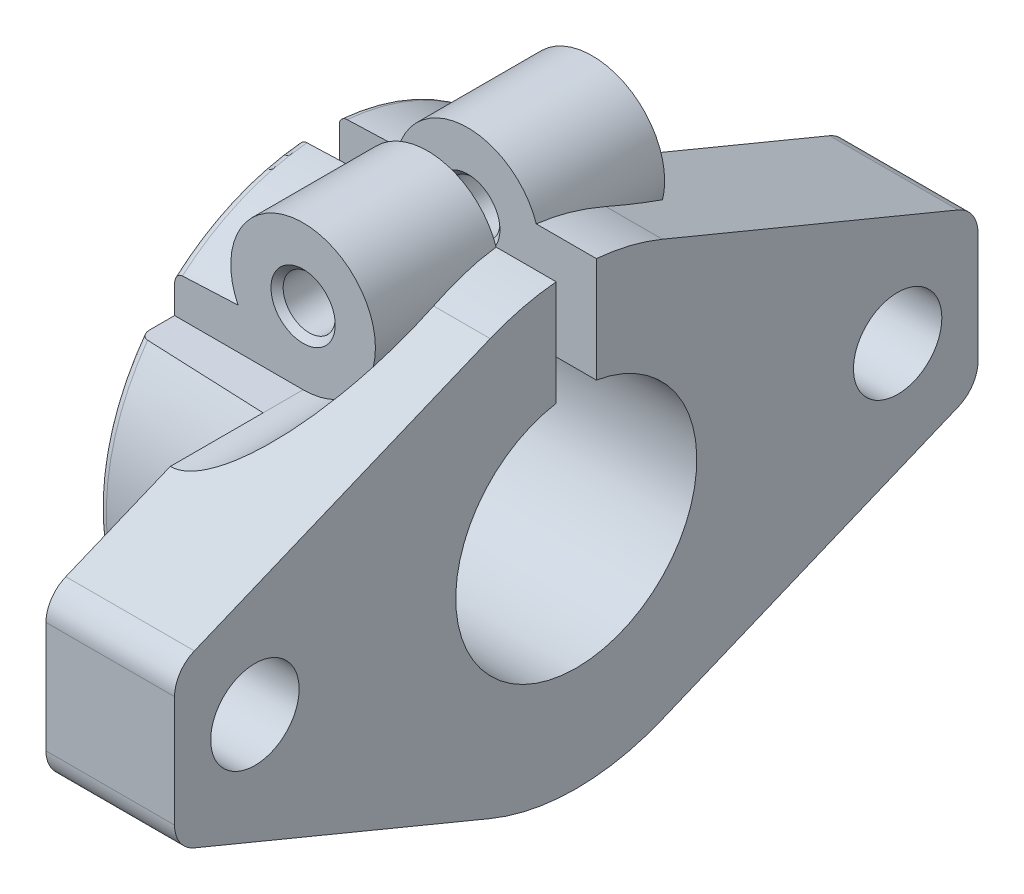
from build123d import *

# Parameters (mm, degrees)
EXTRUDE_1_DEPTH      = 8
EXTRUDE_2_DEPTH      = 9
EXTRUDE_2_DEPTH_BACK = 9
SKETCH_3_R           = 4.5
CUT_EXTRUDE_1_DEPTH  = 9
SKETCH_5_W           = 2.5
SKETCH_5_H           = 31
CUT_EXTRUDE_2_DEPTH  = 16
SKETCH_9_R           = 2.75
CUT_EXTRUDE_3_DEPTH  = 8
SKETCH_10_R          = 2.75
CUT_EXTRUDE_4_DEPTH  = 8


with BuildPart() as part:
    # 草图1 → 凸台-拉伸1 (new body)
    with BuildSketch(Plane(origin=(0, 0, 0), x_dir=(0, 0, -1), z_dir=(1, 0, 0))):
        with BuildLine():
            Line((-25, 3.461794469), (-25, -3.461794469))
            ThreePointArc((-25, -3.461794469), (-24.662939225, -4.572934935), (-23.765366865, -5.309553534))
            Line((-23.765366865, -5.309553534), (-5.357568053, -12.934313455))
            ThreePointArc((-5.357568053, -12.934313455), (-2.731264508, -13.730993926), (0, -14))
            ThreePointArc((0, -14), (2.731264508, -13.730993926), (5.357568053, -12.934313455))
            Line((5.357568053, -12.934313455), (23.765366865, -5.309553534))
            ThreePointArc((23.765366865, -5.309553534), (24.662939225, -4.572934935), (25, -3.461794469))
            Line((25, -3.461794469), (25, 3.461794469))
            ThreePointArc((25, 3.461794469), (24.662939225, 4.572934935), (23.765366865, 5.309553534))
            Line((23.765366865, 5.309553534), (5.357568053, 12.934313455))
            ThreePointArc((5.357568053, 12.934313455), (2.731264508, 13.730993926), (0, 14))
            ThreePointArc((0, 14), (-2.731264508, 13.730993926), (-5.357568053, 12.934313455))
            Line((-5.357568053, 12.934313455), (-23.765366865, 5.309553534))
            ThreePointArc((-23.765366865, 5.309553534), (-24.662939225, 4.572934935), (-25, 3.461794469))
        make_face()
    extrude(amount=-EXTRUDE_1_DEPTH)

    # 草图2 → 旋转1 (revolve)
    with BuildSketch(Plane.XY, mode=Mode.PRIVATE) as revolve_1_sk:
        with BuildLine():
            Line((-16, 0), (-16, 13.230063946))
            ThreePointArc((-16, 13.230063946), (-15.857424619, 13.582950399), (-15.509728944, 13.737754487))
            Line((-15.509728944, 13.737754487), (-8, 14))
            Line((-8, 14), (-8, 0))
            Line((-8, 0), (-16, 0))
        make_face()
    revolve(revolve_1_sk.sketch.rotate(Axis((-8, 0, 0), (-1, 0, 0)), 270), axis=Axis((-8, 0, 0), (-1, 0, 0)))

    # 草图3 → 凸台-拉伸2 (add, two sides: drawn at the far end of the back side and taken through both)
    with BuildSketch(Plane.XY.offset(-EXTRUDE_2_DEPTH_BACK)):
        with Locations((-8, 12.5)):
            Circle(SKETCH_3_R)
    extrude(amount=EXTRUDE_2_DEPTH + EXTRUDE_2_DEPTH_BACK)

    # 草图4 → 切除-拉伸1 (cut)
    with BuildSketch(Plane.XY.offset(9)):
        with BuildLine():
            Line((-16, 8), (-8, 8))
            ThreePointArc((-8, 8), (-4.818019485, 15.681980515), (-12.5, 12.5))
            Line((-12.5, 12.5), (-16, 12.5))
            Line((-16, 12.5), (-16, 8))
        make_face()
    extrude(amount=CUT_EXTRUDE_1_DEPTH, mode=Mode.SUBTRACT)

    # 草图5 → 切除-拉伸2 (cut)
    with BuildSketch(Plane(origin=(0, 0, 0), x_dir=(0, 0, -1), z_dir=(1, 0, 0))):
        with Locations((0, 15.5)):
            Rectangle(SKETCH_5_W, SKETCH_5_H)
    extrude(amount=-CUT_EXTRUDE_2_DEPTH, mode=Mode.SUBTRACT)

    # 草图6 → 切除-旋转1 (revolve, cut)
    with BuildSketch(Plane.XY):
        Polygon((-16, 0), (-16, 10), (-14, 10), (-14, 7.5), (0, 7.5), (0, 0), align=None)
    revolve(axis=Axis((0, 0, 0), (-1, 0, 0)), mode=Mode.SUBTRACT)

    # 草图7 → 切除-旋转2 (revolve, cut)
    with BuildSketch(Plane(origin=(-8, 0, 0), x_dir=(0, 0, -1), z_dir=(1, 0, 0)), mode=Mode.PRIVATE) as cut_revolve_2_sk:
        Polygon((1.25, 12.5), (1.25, 14.5), (1.629, 14.121), (8.621, 14.121), (9.1, 14.6), (13.5, 14.6), (13.5, 12.5), align=None)
    revolve(cut_revolve_2_sk.sketch.rotate(Axis((-8, 12.5, -13.5), (0, 0, 1)), 270), axis=Axis((-8, 12.5, -13.5), (0, 0, 1)), mode=Mode.SUBTRACT)

    # 草图8 → 切除-旋转3 (revolve, cut)
    with BuildSketch(Plane(origin=(-8, 0, 0), x_dir=(0, 0, -1), z_dir=(1, 0, 0)), mode=Mode.PRIVATE) as cut_revolve_3_sk:
        Polygon((-9, 12.5), (-9, 14.5), (-8.621, 14.121), (-1.629, 14.121), (-1.25, 14.5), (-1.25, 12.5), align=None)
    revolve(cut_revolve_3_sk.sketch.rotate(Axis((-8, 12.5, 1.25), (0, 0, 1)), 270), axis=Axis((-8, 12.5, 1.25), (0, 0, 1)), mode=Mode.SUBTRACT)

    # 草图9 → 切除-拉伸3 (cut)
    with BuildSketch(Plane(origin=(0, 0, 0), x_dir=(0, 0, -1), z_dir=(1, 0, 0))):
        with Locations((20, 0)):
            Circle(SKETCH_9_R)
    extrude(amount=-CUT_EXTRUDE_3_DEPTH, mode=Mode.SUBTRACT)

    # 草图10 → 切除-拉伸4 (cut)
    with BuildSketch(Plane(origin=(0, 0, 0), x_dir=(0, 0, -1), z_dir=(1, 0, 0))):
        with Locations((-20, 0)):
            Circle(SKETCH_10_R)
    extrude(amount=-CUT_EXTRUDE_4_DEPTH, mode=Mode.SUBTRACT)


solid = part.part
